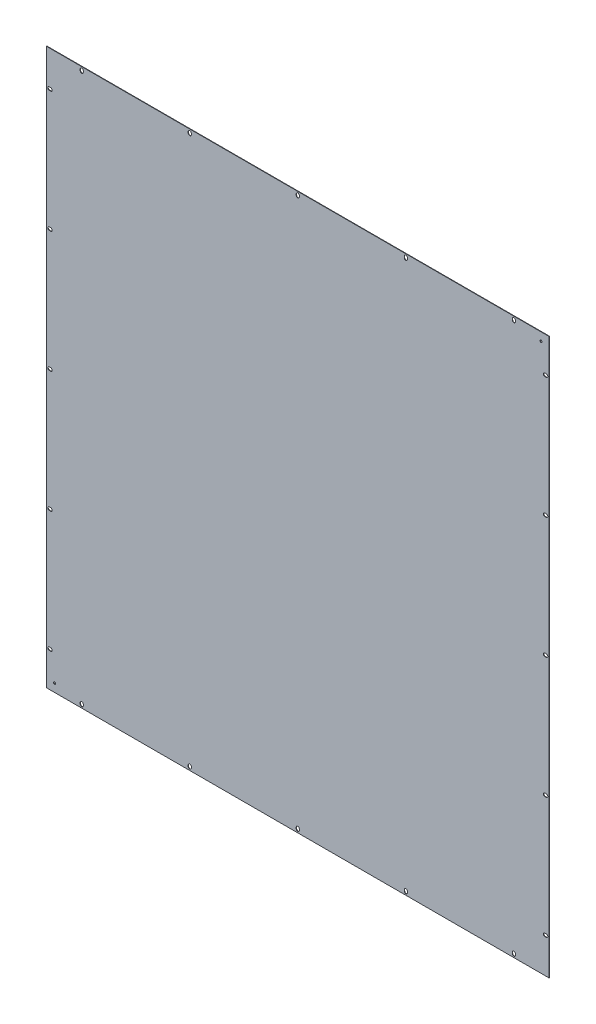
from build123d import *

# Parameters (mm, degrees)
SKETCH_1_W          = 1140
SKETCH_1_H          = 1260
EXTRUDE_1_DEPTH     = 1
SKETCH_3_R          = 2.5
CUT_EXTRUDE_2_DEPTH = 10
CUT_EXTRUDE_3_DEPTH = 10


with BuildPart() as part:
    # 草图1 → 凸台-拉伸1 (new body)
    with BuildSketch(Plane.XY):
        Rectangle(SKETCH_1_W, SKETCH_1_H)
    extrude(amount=EXTRUDE_1_DEPTH)

    # 草图3 → 切除-拉伸2 (cut)
    with BuildSketch(Plane(origin=(0, 0, 0), x_dir=(-1, 0, 0), z_dir=(0, 0, -1))):
        with Locations((551.5, -611.5)):
            Circle(SKETCH_3_R)
        with Locations((-551.5, 611.5)):
            Circle(SKETCH_3_R)
    extrude(amount=-CUT_EXTRUDE_2_DEPTH, mode=Mode.SUBTRACT)

    # 草图4 → 切除-拉伸3 (cut)
    with BuildSketch(Plane(origin=(0, 0, 0), x_dir=(-1, 0, 0), z_dir=(0, 0, -1))):
        with BuildLine():
            Line((3.5, -620.5), (3.5, -623.5))
            ThreePointArc((3.5, -623.5), (0, -627), (-3.5, -623.5))
            Line((-3.5, -623.5), (-3.5, -620.5))
            ThreePointArc((-3.5, -620.5), (0, -617), (3.5, -620.5))
        make_face()
        with BuildLine():
            Line((-241.5, -620.5), (-241.5, -623.5))
            ThreePointArc((-241.5, -623.5), (-245, -627), (-248.5, -623.5))
            Line((-248.5, -623.5), (-248.5, -620.5))
            ThreePointArc((-248.5, -620.5), (-245, -617), (-241.5, -620.5))
        make_face()
        with BuildLine():
            Line((-486.5, -620.5), (-486.5, -623.5))
            ThreePointArc((-486.5, -623.5), (-490, -627), (-493.5, -623.5))
            Line((-493.5, -623.5), (-493.5, -620.5))
            ThreePointArc((-493.5, -620.5), (-490, -617), (-486.5, -620.5))
        make_face()
        with BuildLine():
            Line((486.5, -620.5), (486.5, -623.5))
            ThreePointArc((486.5, -623.5), (490, -627), (493.5, -623.5))
            Line((493.5, -623.5), (493.5, -620.5))
            ThreePointArc((493.5, -620.5), (490, -617), (486.5, -620.5))
        make_face()
        with BuildLine():
            Line((241.5, -620.5), (241.5, -623.5))
            ThreePointArc((241.5, -623.5), (245, -627), (248.5, -623.5))
            Line((248.5, -623.5), (248.5, -620.5))
            ThreePointArc((248.5, -620.5), (245, -617), (241.5, -620.5))
        make_face()
        with BuildLine():
            Line((-560.5, -3.5), (-563.5, -3.5))
            ThreePointArc((-563.5, -3.5), (-567, 0), (-563.5, 3.5))
            Line((-563.5, 3.5), (-560.5, 3.5))
            ThreePointArc((-560.5, 3.5), (-557, 0), (-560.5, -3.5))
        make_face()
        with BuildLine():
            Line((-560.5, 271.5), (-563.5, 271.5))
            ThreePointArc((-563.5, 271.5), (-567, 275), (-563.5, 278.5))
            Line((-563.5, 278.5), (-560.5, 278.5))
            ThreePointArc((-560.5, 278.5), (-557, 275), (-560.5, 271.5))
        make_face()
        with BuildLine():
            Line((-560.5, 546.5), (-563.5, 546.5))
            ThreePointArc((-563.5, 546.5), (-567, 550), (-563.5, 553.5))
            Line((-563.5, 553.5), (-560.5, 553.5))
            ThreePointArc((-560.5, 553.5), (-557, 550), (-560.5, 546.5))
        make_face()
        with BuildLine():
            Line((-560.5, -546.5), (-563.5, -546.5))
            ThreePointArc((-563.5, -546.5), (-567, -550), (-563.5, -553.5))
            Line((-563.5, -553.5), (-560.5, -553.5))
            ThreePointArc((-560.5, -553.5), (-557, -550), (-560.5, -546.5))
        make_face()
        with BuildLine():
            Line((-560.5, -271.5), (-563.5, -271.5))
            ThreePointArc((-563.5, -271.5), (-567, -275), (-563.5, -278.5))
            Line((-563.5, -278.5), (-560.5, -278.5))
            ThreePointArc((-560.5, -278.5), (-557, -275), (-560.5, -271.5))
        make_face()
        with BuildLine():
            Line((241.5, 620.5), (241.5, 623.5))
            ThreePointArc((241.5, 623.5), (245, 627), (248.5, 623.5))
            Line((248.5, 623.5), (248.5, 620.5))
            ThreePointArc((248.5, 620.5), (245, 617), (241.5, 620.5))
        make_face()
        with BuildLine():
            Line((486.5, 620.5), (486.5, 623.5))
            ThreePointArc((486.5, 623.5), (490, 627), (493.5, 623.5))
            Line((493.5, 623.5), (493.5, 620.5))
            ThreePointArc((493.5, 620.5), (490, 617), (486.5, 620.5))
        make_face()
        with BuildLine():
            Line((-486.5, 620.5), (-486.5, 623.5))
            ThreePointArc((-486.5, 623.5), (-490, 627), (-493.5, 623.5))
            Line((-493.5, 623.5), (-493.5, 620.5))
            ThreePointArc((-493.5, 620.5), (-490, 617), (-486.5, 620.5))
        make_face()
        with BuildLine():
            Line((-241.5, 620.5), (-241.5, 623.5))
            ThreePointArc((-241.5, 623.5), (-245, 627), (-248.5, 623.5))
            Line((-248.5, 623.5), (-248.5, 620.5))
            ThreePointArc((-248.5, 620.5), (-245, 617), (-241.5, 620.5))
        make_face()
        with BuildLine():
            Line((3.5, 620.5), (3.5, 623.5))
            ThreePointArc((3.5, 623.5), (0, 627), (-3.5, 623.5))
            Line((-3.5, 623.5), (-3.5, 620.5))
            ThreePointArc((-3.5, 620.5), (0, 617), (3.5, 620.5))
        make_face()
        with BuildLine():
            Line((560.5, 546.5), (563.5, 546.5))
            ThreePointArc((563.5, 546.5), (567, 550), (563.5, 553.5))
            Line((563.5, 553.5), (560.5, 553.5))
            ThreePointArc((560.5, 553.5), (557, 550), (560.5, 546.5))
        make_face()
        with BuildLine():
            Line((560.5, -271.5), (563.5, -271.5))
            ThreePointArc((563.5, -271.5), (567, -275), (563.5, -278.5))
            Line((563.5, -278.5), (560.5, -278.5))
            ThreePointArc((560.5, -278.5), (557, -275), (560.5, -271.5))
        make_face()
        with BuildLine():
            Line((560.5, -546.5), (563.5, -546.5))
            ThreePointArc((563.5, -546.5), (567, -550), (563.5, -553.5))
            Line((563.5, -553.5), (560.5, -553.5))
            ThreePointArc((560.5, -553.5), (557, -550), (560.5, -546.5))
        make_face()
        with BuildLine():
            Line((560.5, 271.5), (563.5, 271.5))
            ThreePointArc((563.5, 271.5), (567, 275), (563.5, 278.5))
            Line((563.5, 278.5), (560.5, 278.5))
            ThreePointArc((560.5, 278.5), (557, 275), (560.5, 271.5))
        make_face()
        with BuildLine():
            Line((560.5, -3.5), (563.5, -3.5))
            ThreePointArc((563.5, -3.5), (567, 0), (563.5, 3.5))
            Line((563.5, 3.5), (560.5, 3.5))
            ThreePointArc((560.5, 3.5), (557, 0), (560.5, -3.5))
        make_face()
    extrude(amount=-CUT_EXTRUDE_3_DEPTH, mode=Mode.SUBTRACT)


solid = part.part
